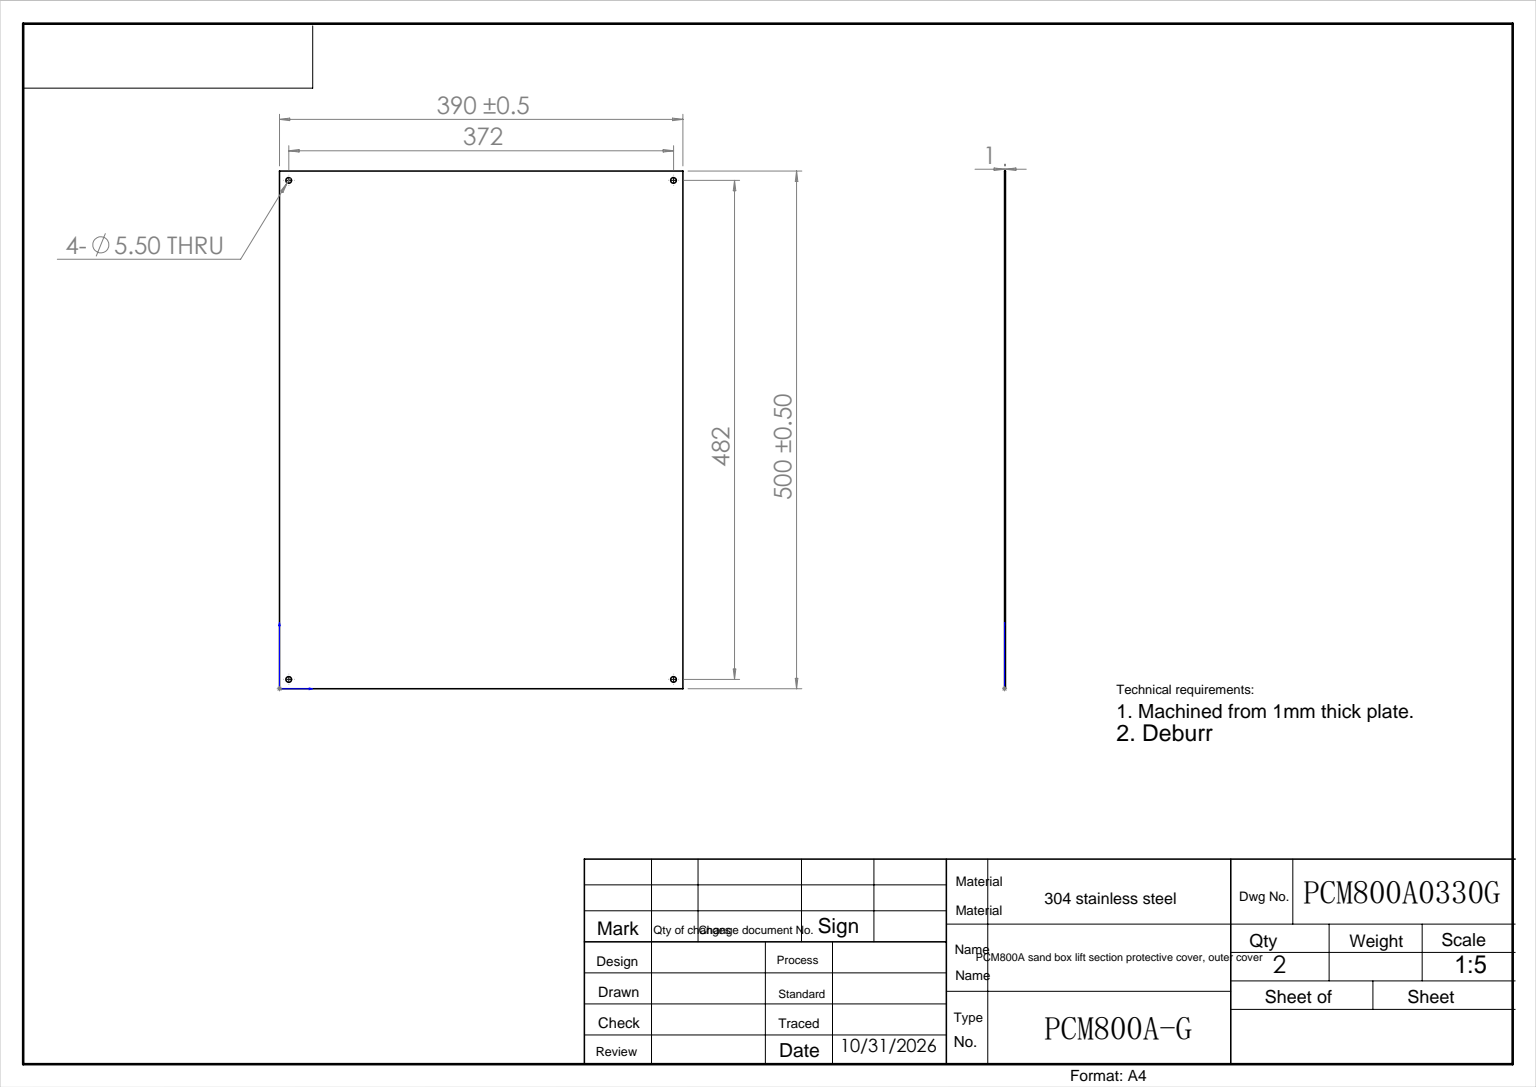
SolidWorks part; units mm, degrees
ref_plane "前视基准面" through (0, 0, 0) normal (0, 0, 1) x (1, 0, 0)
ref_plane "上视基准面" through (0, 0, 0) normal (0, 1, 0) x (1, 0, 0)
ref_plane "右视基准面" through (0, 0, 0) normal (1, 0, 0) x (0, 0, -1)
sketch "草图1" plane through (0, 0, 0) normal (0, 0, 1) x (1, 0, 0)
  line L1 (0, 0) -> (390, 0)
  line L2 (0, 0) -> (0, 500)
  line L3 (0, 500) -> (390, 500)
  line L4 (390, 0) -> (390, 500)
  dimension "D1" = 390
  dimension "D2" = 500
extrude "凸台-拉伸1" add sketch "草图1" along normal blind 1
sketch "草图2" plane through (0, 0, 1) normal (0, 0, 1) x (1, 0, 0)
  line L0 (0, 250) -> (527.7164, 250) construction
  line L1 (0, 500) -> (0, 0) construction
  line L2 (195, 500) -> (195, -71.2266) construction
  line L3 (390, 500) -> (0, 500) construction
  circle A0 centre (9, 491) radius 2.75
  circle A1 centre (381, 491) radius 2.75
  circle A2 centre (9, 9) radius 2.75
  circle A3 centre (381, 9) radius 2.75
  dimension "D1" = 5.5
  dimension "D2" = 5.5
  dimension "D3" = 5.5
  dimension "D4" = 5.5
  dimension "D5" = 372
  dimension "D6" = 482
  dimension "D7" = 241
  dimension "D8" = 186
  dimension "D9" = 482
  dimension "D10" = 241
  dimension "D11" = 372
  dimension "D12" = 186
extrude "切除-拉伸1" cut sketch "草图2" against normal blind 1
